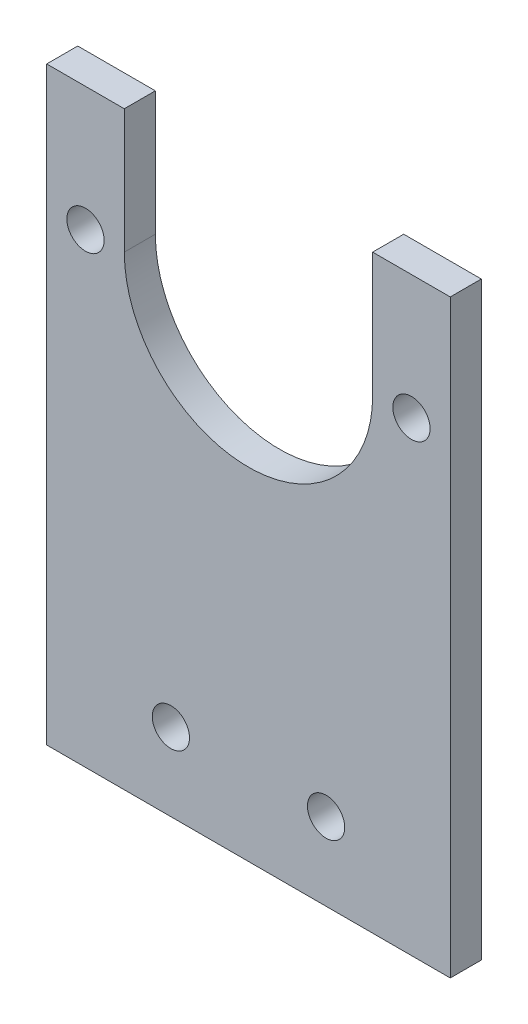
from build123d import *

# Parameters (mm, degrees)
SKETCH_1_R      = 6
EXTRUDE_1_DEPTH = 10


with BuildPart() as part:
    # 草图1 → 凸台-拉伸1 (new body)
    with BuildSketch(Plane.XY):
        with BuildLine():
            Line((0, 0), (130, 0))
            Line((130, 0), (130, 190))
            Line((130, 190), (105, 190))
            Line((105, 190), (105, 150))
            ThreePointArc((105, 150), (65, 110), (25, 150))
            Line((25, 150), (25, 190))
            Line((25, 190), (0, 190))
            Line((0, 190), (0, 0))
        make_face()
        with Locations((117.5, 150)):
            Circle(SKETCH_1_R, mode=Mode.SUBTRACT)
        with Locations((12.5, 150)):
            Circle(SKETCH_1_R, mode=Mode.SUBTRACT)
        with Locations((40, 25)):
            Circle(SKETCH_1_R, mode=Mode.SUBTRACT)
        with Locations((90, 25)):
            Circle(SKETCH_1_R, mode=Mode.SUBTRACT)
    extrude(amount=EXTRUDE_1_DEPTH)


solid = part.part
